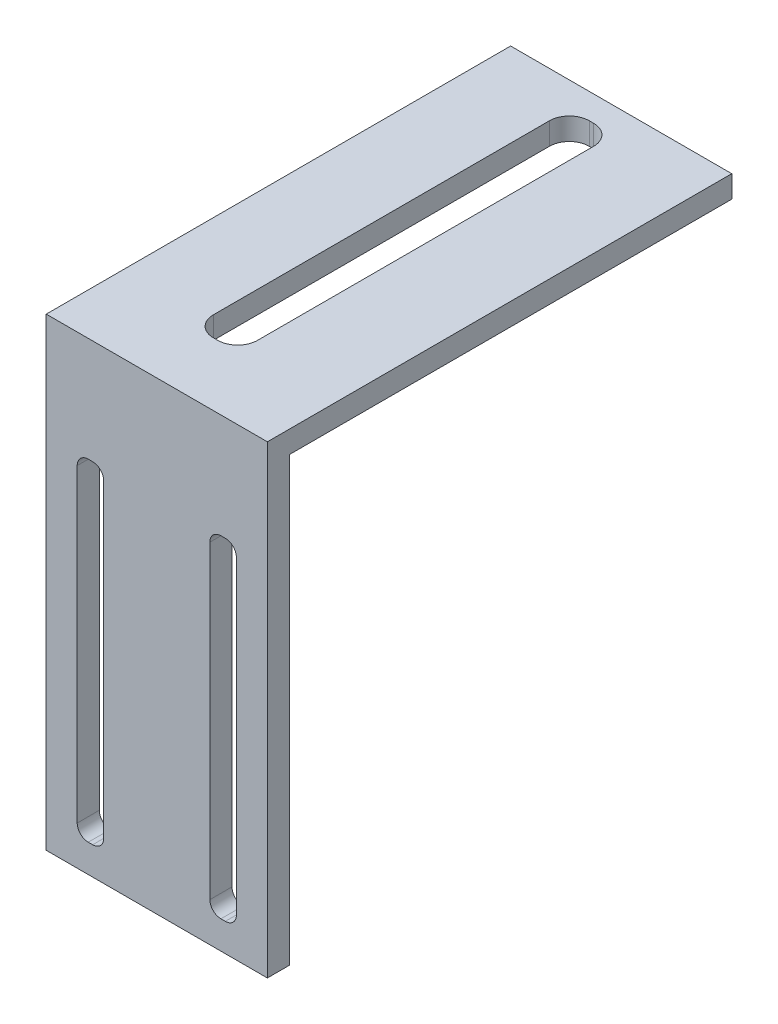
SolidWorks part; units mm, degrees
material "PVC Rigid"
ref_plane "Front Plane" through (0, 0, 0) normal (0, 0, 1) x (1, 0, 0)
ref_plane "Top Plane" through (0, 0, 0) normal (0, 1, 0) x (1, 0, 0)
ref_plane "Right Plane" through (0, 0, 0) normal (1, 0, 0) x (0, 0, -1)
sketch "Sketch1" plane through (0, 0, 0) normal (0, 0, 1) x (1, 0, 0)
  line L1 (25, -50) -> (-25, -50)
  line L2 (25, -50) -> (25, 50)
  line L3 (25, 50) -> (-25, 50)
  line L4 (-25, -50) -> (-25, 50)
  line L5 (25, -50) -> (-25, 50) construction
  line L6 (25, 50) -> (-25, -50) construction
  point P0 (0, 0)
  dimension "D1" = 100
  dimension "D2" = 50
extrude "Boss-Extrude1" add sketch "Sketch1" along normal blind 5
sketch "Sketch2" plane through (0, 0, 5) normal (0, 0, 1) x (1, 0, 0)
  line L0 (0, 32.1879) -> (0, -24.1157) construction
  line L1 (-15, 24.3175) -> (-15, -24.1157) construction
  line L2 (15, 24.3175) -> (15, -24.1157) construction
  line L4 (-14.5, -43.6551) -> (-15.5, -43.6551)
  line L5 (-12, -41.1551) -> (-12, 28.8449)
  line L6 (-14.5, 31.3449) -> (-15.5, 31.3449)
  line L7 (-18, -41.1551) -> (-18, 28.8449)
  line L8 (-12, -43.6551) -> (-18, 31.3449) construction
  line L9 (-12, 31.3449) -> (-18, -43.6551) construction
  line L10 (15.5, -43.6551) -> (14.5, -43.6551)
  line L11 (18, -41.1551) -> (18, 28.8449)
  line L12 (15.5, 31.3449) -> (14.5, 31.3449)
  line L13 (12, -41.1551) -> (12, 28.8449)
  line L14 (18, -43.6551) -> (12, 31.3449) construction
  line L15 (18, 31.3449) -> (12, -43.6551) construction
  arc A0 (14.5, 31.3449) -> (12, 28.8449) centre (14.5, 28.8449) ccw
  arc A1 (18, 28.8449) -> (15.5, 31.3449) centre (15.5, 28.8449) ccw
  arc A2 (14.5, -43.6551) -> (12, -41.1551) centre (14.5, -41.1551) cw
  arc A3 (15.5, -43.6551) -> (18, -41.1551) centre (15.5, -41.1551) ccw
  arc A4 (-15.5, -43.6551) -> (-18, -41.1551) centre (-15.5, -41.1551) cw
  arc A5 (-14.5, -43.6551) -> (-12, -41.1551) centre (-14.5, -41.1551) ccw
  arc A6 (-12, 28.8449) -> (-14.5, 31.3449) centre (-14.5, 28.8449) ccw
  arc A7 (-15.5, 31.3449) -> (-18, 28.8449) centre (-15.5, 28.8449) ccw
  point P7 (-15, -6.1551)
  point P12 (15, -6.1551)
  dimension "D7" = 2.5
  dimension "D1" = 15
  dimension "D2" = 15
  dimension "D3" = 6
  dimension "D4" = 6
  dimension "D5" = 75
  dimension "D6" = 75
extrude "Cut-Extrude1" cut sketch "Sketch2" against normal blind 10
sketch "Sketch4" plane through (0, 0, 0) normal (0, 0, -1) x (-1, 0, 0)
  line L0 (-25, 50) -> (-25, 55)
  line L1 (25, 50) -> (25, 55)
  line L2 (25, 55) -> (-25, 55)
  line L3 (25, 50) -> (-25, 50)
  dimension "D1" = 5
extrude "Boss-Extrude2" add sketch "Sketch4" along normal blind 100 and the other way blind 5
sketch "Sketch5" plane through (0, 50, 0) normal (0, -1, 0) x (1, 0, 0)
  line L1 (-0.474, -94.2529) -> (-1.474, -94.2529)
  line L2 (4.026, -89.7529) -> (4.026, -13.7529)
  line L3 (-0.474, -9.2529) -> (-1.474, -9.2529)
  line L4 (-5.974, -89.7529) -> (-5.974, -13.7529)
  line L5 (4.026, -94.2529) -> (-5.974, -9.2529) construction
  line L6 (4.026, -9.2529) -> (-5.974, -94.2529) construction
  arc A0 (-1.474, -94.2529) -> (-5.974, -89.7529) centre (-1.474, -89.7529) cw
  arc A1 (-0.474, -94.2529) -> (4.026, -89.7529) centre (-0.474, -89.7529) ccw
  arc A2 (4.026, -13.7529) -> (-0.474, -9.2529) centre (-0.474, -13.7529) ccw
  arc A3 (-1.474, -9.2529) -> (-5.974, -13.7529) centre (-1.474, -13.7529) ccw
  point P0 (-0.974, -51.7529)
  dimension "D3" = 4.5
  dimension "D1" = 10
  dimension "D2" = 85
extrude "Cut-Extrude3" cut sketch "Sketch5" against normal blind 80
